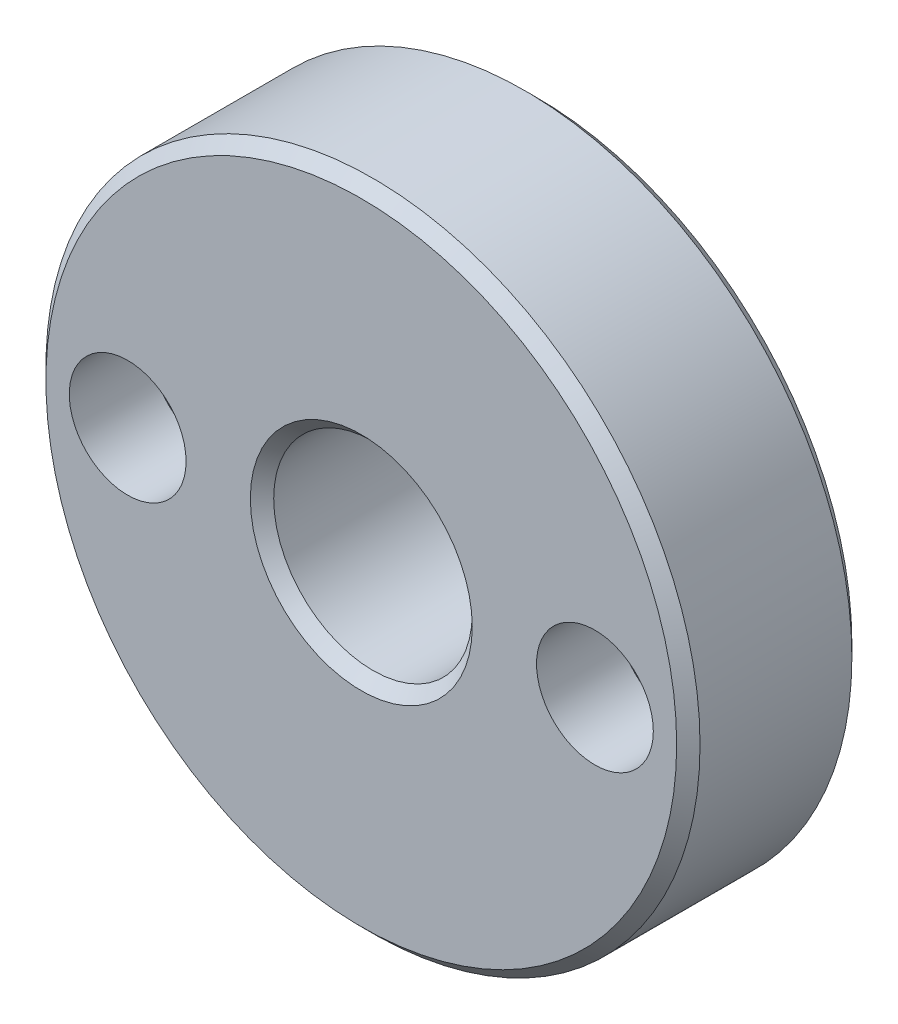
from build123d import *

# Parameters (mm, degrees)
SKETCH1_R           = 28
BOSS_EXTRUDE1_DEPTH = 15
HOLE1_D             = 17
HOLE2_D             = 5.5
HOLE2_CBORE_D       = 10
HOLE2_CBORE_DEPTH   = 7
CHAMFER1_SIZE       = 1


with BuildPart() as part:
    # Sketch1 → Boss-Extrude1 (new body)
    with BuildSketch(Plane.XY):
        Circle(SKETCH1_R)
    extrude(amount=BOSS_EXTRUDE1_DEPTH)

    # Hole1 (through all)
    with Locations(Plane.XY.offset(15)):
        with Locations((0, 0)):
            Hole(HOLE1_D / 2)

    # Hole2 (through all)
    with Locations(Plane.XY.offset(15)):
        with Locations((-20, 0), (20, 0)):
            CounterBoreHole(HOLE2_D / 2, HOLE2_CBORE_D / 2, HOLE2_CBORE_DEPTH)

    # Chamfer1
    chamfer1_edges = [part.edges().sort_by_distance(p)[0] for p in [
        (-28, 0, 0),
        (-28, 0, 15),
        (8.5, 0, 15),
        (8.5, 0, 0),
    ]]
    chamfer(chamfer1_edges, length=CHAMFER1_SIZE)


solid = part.part
